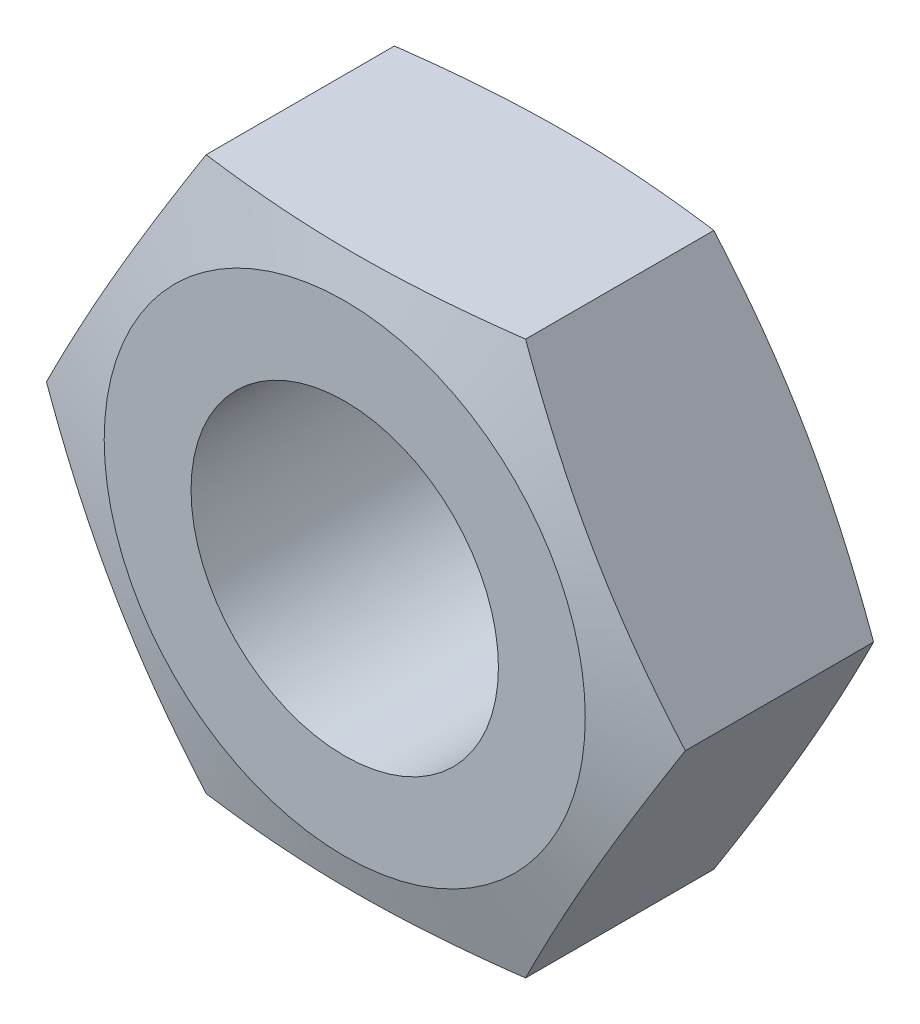
from build123d import *

# Parameters (mm, degrees)
SKETCH1_R           = 10
BOSS_EXTRUDE1_DEPTH = 15


with BuildPart() as part:
    # Sketch1 → Boss-Extrude1 (new body)
    with BuildSketch(Plane.XY):
        Polygon((-20.784609691, 0), (-10.392304845, -18), (10.392304845, -18), (20.784609691, 0), (10.392304845, 18), (-10.392304845, 18), align=None)
        Circle(SKETCH1_R, mode=Mode.SUBTRACT)
    extrude(amount=BOSS_EXTRUDE1_DEPTH)

    # Sketch2 → Cut-Revolve1 (revolve, cut)
    with BuildSketch(Plane(origin=(0, 0, 0), x_dir=(1, 0, 0), z_dir=(0, 1, 0))):
        Polygon((13.784609691, 0.5), (25.784609691, -2.715390309), (25.784609691, 0.5), align=None)
        Polygon((25.784609691, -15.5), (25.784609691, -12.284609691), (13.784609691, -15.5), align=None)
    revolve(axis=Axis((0, 0, 15), (0, 0, -1)), mode=Mode.SUBTRACT)


solid = part.part
